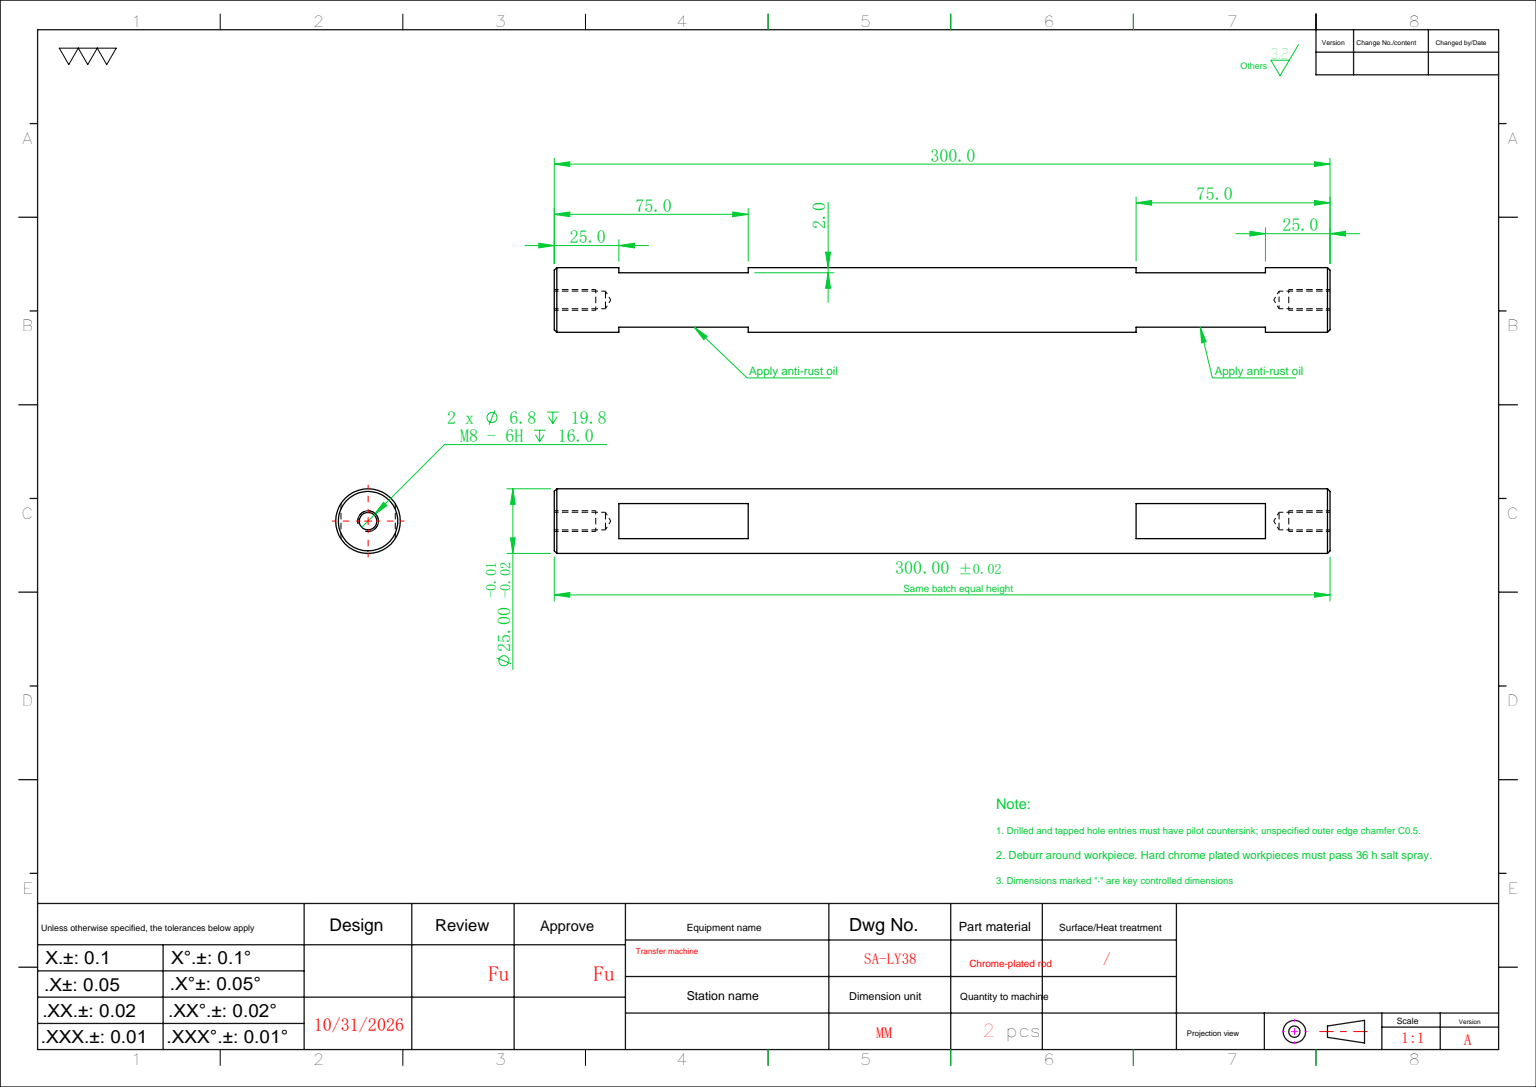
SolidWorks part; units mm, degrees
ref_plane "前视基准面" through (0, 0, 0) normal (0, 0, 1) x (1, 0, 0)
ref_plane "上视基准面" through (0, 0, 0) normal (0, 1, 0) x (1, 0, 0)
ref_plane "右视基准面" through (0, 0, 0) normal (1, 0, 0) x (0, 0, -1)
sketch "草图1" plane through (0, 0, 0) normal (0, 0, 1) x (1, 0, 0)
  circle A0 centre (0, 0) radius 12.5
  dimension "D1" = 25
extrude "凸台-拉伸1" add sketch "草图1" along normal mid plane 300
sketch "草图2" plane through (0, 0, 0) normal (1, 0, 0) x (0, 0, -1)
  line L0 (150, 12.5) -> (-150, 12.5) construction
  line L1 (-125, 12.5) -> (-75, 12.5)
  line L2 (-125, 12.5) -> (-125, 10.5)
  line L3 (-125, 10.5) -> (-75, 10.5)
  line L4 (-75, 12.5) -> (-75, 10.5)
  line L5 (0, -12.5) -> (0, 12.5) construction
  line L6 (-150, -12.5) -> (150, -12.5) construction
  line L7 (0, 0) -> (-335.9133, 0) construction
  line L8 (-75, -12.5) -> (-75, -10.5)
  line L9 (-125, -10.5) -> (-75, -10.5)
  line L10 (-125, -12.5) -> (-125, -10.5)
  line L11 (-125, -12.5) -> (-75, -12.5)
  line L12 (125, -12.5) -> (75, -12.5)
  line L13 (125, -12.5) -> (125, -10.5)
  line L14 (125, -10.5) -> (75, -10.5)
  line L15 (75, -12.5) -> (75, -10.5)
  line L16 (75, 12.5) -> (75, 10.5)
  line L17 (125, 10.5) -> (75, 10.5)
  line L18 (125, 12.5) -> (125, 10.5)
  line L19 (125, 12.5) -> (75, 12.5)
  dimension "D1" = 2
  dimension "D2" = 50
  dimension "D3" = 150
extrude "切除-拉伸1" cut sketch "草图2" against normal mid plane 200
chamfer "倒角1" distance 1 angle 45 2 edges at (12.5, 0, 150) (12.5, 0, -150)
hole_wizard "M8 螺纹孔1" positions "草图3" profile "草图4" tap size "M8" standard "ISO"
sketch "草图3" plane through (0, 0, -150) normal (0, 0, -1) x (-1, 0, 0)
  point P0 (0, 0)
cosmetic thread "孔螺蚊线1" parameters "D1"=16, "D2"=8
sketch "草图4" plane through (0, 0, -150) normal (1, 0, 0) x (0, 1, 0)
  line L0 (0, 0) -> (0, 21.7929)
  line L1 (0, 21.7929) -> (3.4, 19.75)
  line L2 (3.4, 19.75) -> (3.4, 0)
  line L5 (3.4, 0) -> (0, 0)
  line L10 (0, 21.7929) -> (-3.4, 19.75) construction
  line L11 (0, -6.35) -> (0, 107.95) construction
  dimension "螺纹孔钻头直径" = 6.8
  dimension "螺纹孔钻头深度" = 19.75
  dimension "导头角度" = 118
mirror "镜向1" about plane through (0, 0, 0) normal (0, 0, 1) of "M8 螺纹孔1"
cosmetic thread "孔螺蚊线2"
